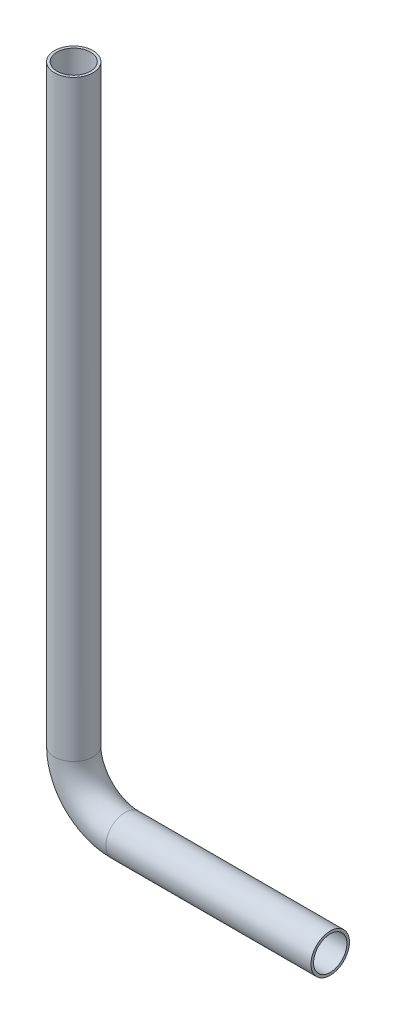
from build123d import *

# Parameters (mm, degrees)
SWEEP_THIN1_PROFILE_R   = 15
SWEEP_THIN1_PROFILE_R_2 = 13


with BuildPart() as part:
    # Sweep-Thin1: sweep along a path in Sketch1
    with BuildLine(Plane.XY) as sweep_thin1_path:
        Line((200, 0), (40, 0))
        ThreePointArc((40, 0), (11.715728753, 11.715728753), (0, 40))
        Line((0, 40), (0, 502))
    # Sweep-Thin1 profile (on start of the path) → Sweep-Thin1 (sweep)
    with BuildSketch(Plane(origin=(200, 0, 0), x_dir=(0, 0, -1), z_dir=(-1, 0, 0))):
        Circle(SWEEP_THIN1_PROFILE_R)
        Circle(SWEEP_THIN1_PROFILE_R_2, mode=Mode.SUBTRACT)
    sweep(path=sweep_thin1_path.line)


solid = part.part
